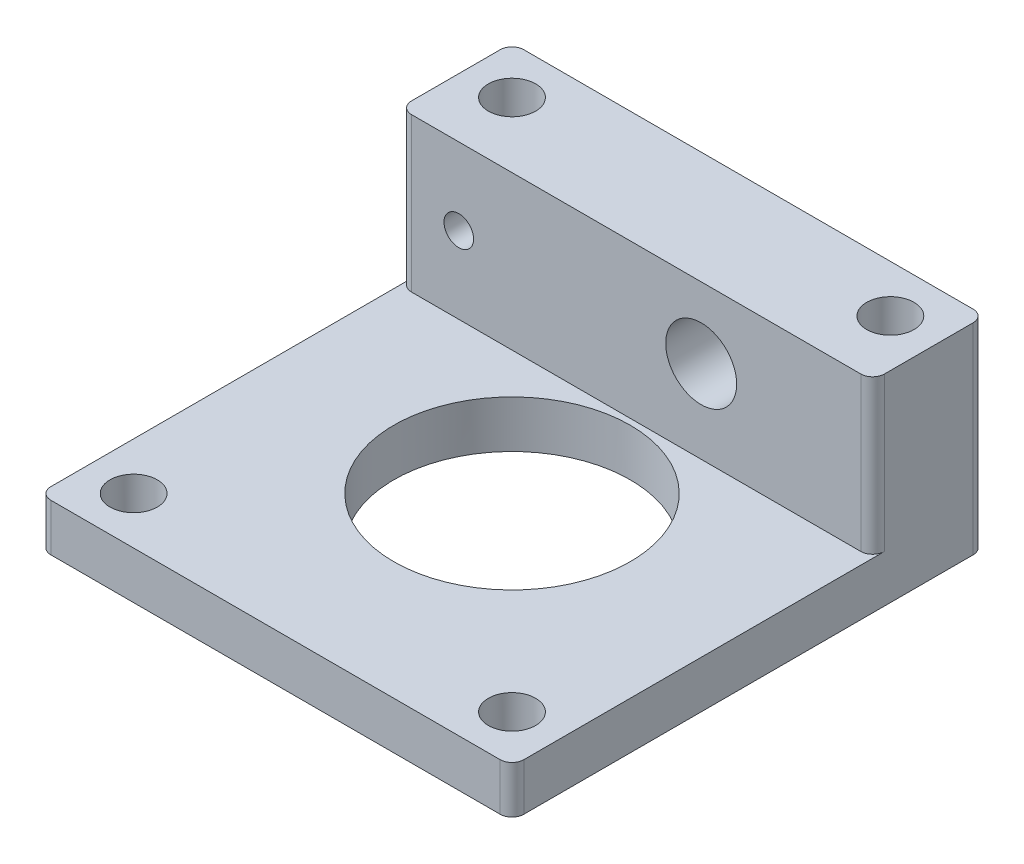
SolidWorks part; units mm, degrees
material "Brass"
ref_plane "Front Plane" through (0, 0, 0) normal (0, 0, 1) x (1, 0, 0)
ref_plane "Top Plane" through (0, 0, 0) normal (0, 1, 0) x (1, 0, 0)
ref_plane "Right Plane" through (0, 0, 0) normal (1, 0, 0) x (0, 0, -1)
sketch "Sketch1" plane through (0, 0, 0) normal (1, 0, 0) x (0, 0, -1)
  line L1 (0, 0) -> (40, 0)
  line L2 (0, 0) -> (0, 4)
  line L3 (0, 4) -> (30.5, 4)
  line L4 (40, 0) -> (40, 4)
  line L6 (40, 4) -> (40, 17)
  line L7 (40, 17) -> (30.5, 17)
  line L8 (30.5, 4) -> (30.5, 17)
  dimension "D1" = 40
  dimension "D2" = 17
  dimension "D3" = 4
  dimension "D4" = 9.5
extrude "Boss-Extrude1" add sketch "Sketch1" along normal mid plane 40
sketch "Sketch2" plane through (0, 4, 0) normal (0, 1, 0) x (1, 0, 0)
  line L0 (20, 0) -> (-20, 0) construction
  line L1 (0, 20) -> (20, 40) construction
  circle A0 centre (0, 20) radius 10
  circle A1 centre (16, 36) radius 2
  circle A2 centre (16, 4) radius 2
  circle A3 centre (-16, 4) radius 2
  circle A4 centre (-16, 36) radius 2
  point P17 (0, 20)
  dimension "D2" = 20
  dimension "D3" = 4
  dimension "D4" = 16
  dimension "D1" = 20
  dimension "D5" = 4
extrude "Cut-Extrude1" cut sketch "Sketch2" against normal through all and the other way through all
fillet "Fillet1" radius 1 6 edges at (-20, 2, 0) (20, 2, 0) (-20, 8.5, -40) (20, 8.5, -40) (-20, 10.5, -30.5) (20, 10.5, -30.5)
sketch "Sketch3" plane through (0, 0, -30.5) normal (0, 0, 1) x (1, 0, 0)
  line L0 (-20, 4) -> (-20, 17) construction
  line L1 (20, 17) -> (20, 4) construction
  line L2 (19, 17) -> (-19, 17) construction
  circle A0 centre (5.5, 11) radius 3
  circle A1 centre (-15, 10.5) radius 1.25
  dimension "D1" = 5
  dimension "D2" = 14.5
  dimension "D3" = 6
  dimension "D4" = 6.5
  dimension "D5" = 6
  dimension "D6" = 2.5
extrude "Cut-Extrude2" cut sketch "Sketch3" against normal through all
